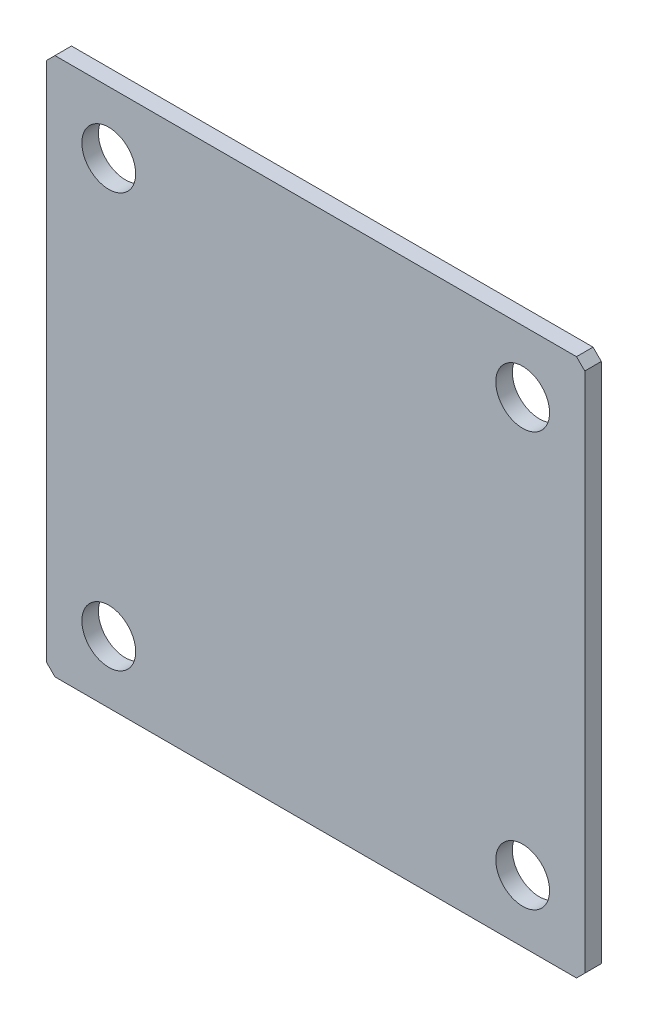
from build123d import *

# Parameters (mm, degrees)
SKETCH_1_W              = 130
SKETCH_1_H              = 130
EXTRUDE_1_DEPTH         = 4
CHAMFER_1_SIZE          = 2
HOLE_WIZARD_13_0_13_1_D = 13


with BuildPart() as part:
    # 草图1 → 凸台-拉伸1 (new body)
    with BuildSketch(Plane.XY):
        with Locations((-65, 0)):
            Rectangle(SKETCH_1_W, SKETCH_1_H)
    extrude(amount=EXTRUDE_1_DEPTH)

    # 倒角1
    chamfer_1_edges = [part.edges().sort_by_distance(p)[0] for p in [
        (0, -65, 2),
        (-130, -65, 2),
        (-130, 65, 2),
        (0, 65, 2),
    ]]
    chamfer(chamfer_1_edges, length=CHAMFER_1_SIZE)

    # Ø13.0 (13) 直径孔1 (through all)
    with Locations(Plane(origin=(0, 0, 0), x_dir=(-1, 0, 0), z_dir=(0, 0, -1))):
        with Locations((15, -50), (15, 50), (115, -50), (115, 50)):
            Hole(HOLE_WIZARD_13_0_13_1_D / 2)


solid = part.part
